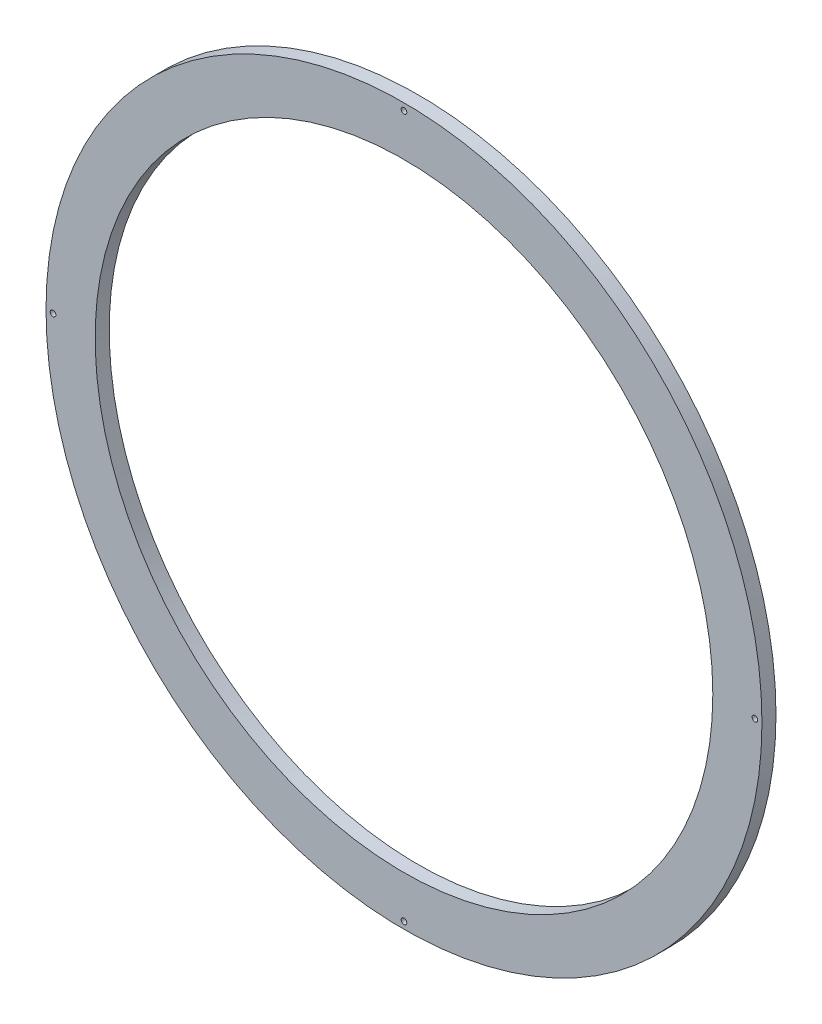
SolidWorks part; units mm, degrees
ref_plane "Front Plane" through (0, 0, 0) normal (0, 0, 1) x (1, 0, 0)
ref_plane "Top Plane" through (0, 0, 0) normal (0, 1, 0) x (1, 0, 0)
ref_plane "Right Plane" through (0, 0, 0) normal (1, 0, 0) x (0, 0, -1)
sketch "Sketch1" plane through (0, 0, 0) normal (0, 0, 1) x (1, 0, 0)
  circle A1 centre (0, 0) radius 110
  circle A2 centre (0, 0) radius 127.5
  dimension "D2" = 220
  dimension "D3" = 255
extrude "Boss-Extrude1" add sketch "Sketch1" along normal blind 5
sketch "Sketch4" plane through (0, 0, 5) normal (0, 0, 1) x (1, 0, 0)
  circle A2 centre (0, 125) radius 1
  dimension "D2" = 2
extrude "Cut-Extrude2" cut sketch "Sketch4" against normal blind 5
pattern_circular "CirPattern2" count 4 over 360 about axis through (0, 0, 0) along (0, 0, 1) of "Cut-Extrude2"
